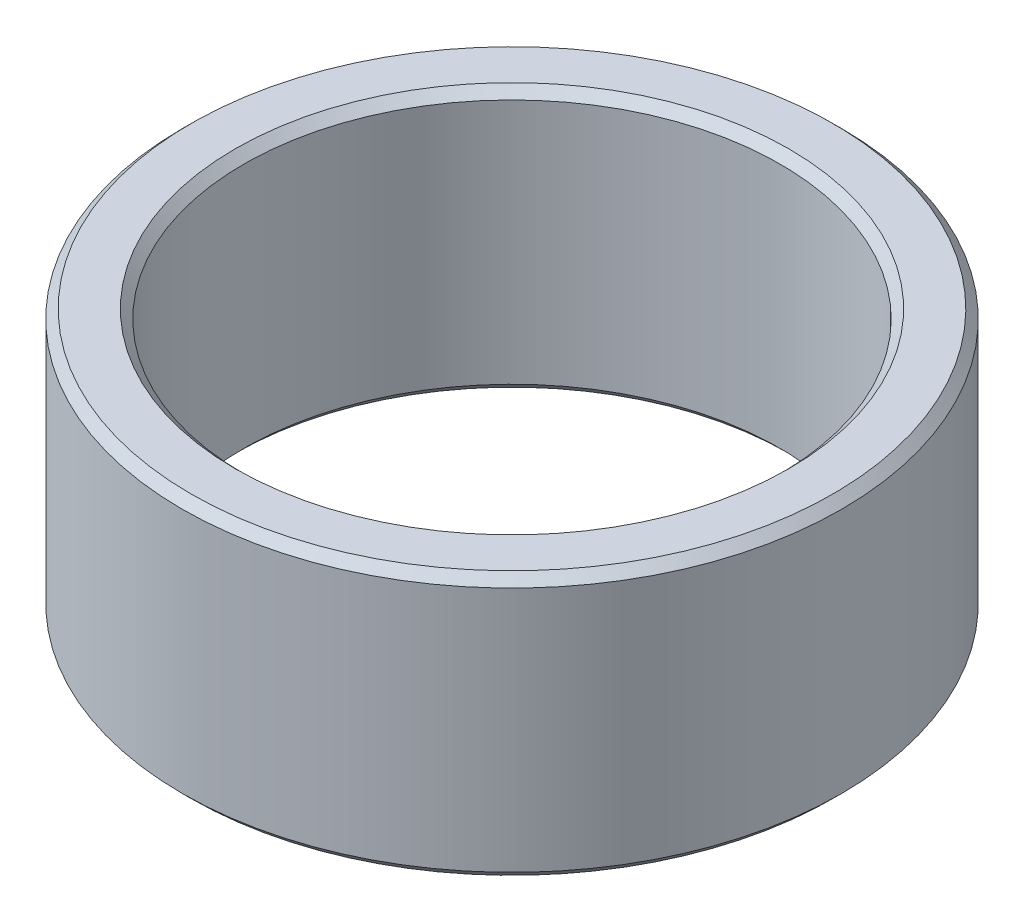
from build123d import *

# Parameters (mm, degrees)
SKETCH1_R           = 37.5
SKETCH1_R_2         = 30.5
BOSS_EXTRUDE1_DEPTH = 30
CHAMFER1_SIZE       = 1


with BuildPart() as part:
    # Sketch1 → Boss-Extrude1 (new body)
    with BuildSketch(Plane(origin=(0, 0, 0), x_dir=(1, 0, 0), z_dir=(0, 1, 0))):
        with Locations(Location((0, 0, 0), (0, 0, 270))):
            Circle(SKETCH1_R)
        with Locations(Location((0, 0, 0), (0, 0, 270))):
            Circle(SKETCH1_R_2, mode=Mode.SUBTRACT)
    extrude(amount=BOSS_EXTRUDE1_DEPTH)

    # Chamfer1
    chamfer1_edges = [part.edges().sort_by_distance(p)[0] for p in [
        (0, 0, -37.5),
        (0, 30, -37.5),
        (0, 0, -30.5),
        (0, 30, -30.5),
    ]]
    chamfer(chamfer1_edges, length=CHAMFER1_SIZE)


solid = part.part
